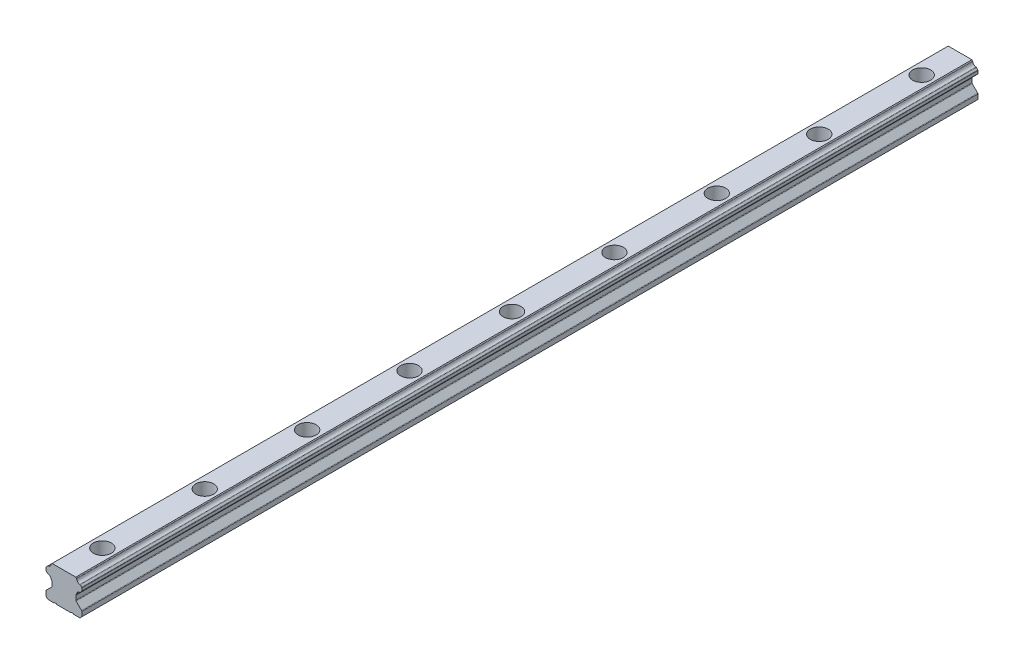
SolidWorks part; units mm, degrees
ref_plane "前视基准面" through (0, 0, 0) normal (0, 0, 1) x (1, 0, 0)
ref_plane "上视基准面" through (0, 0, 0) normal (0, 1, 0) x (1, 0, 0)
ref_plane "右视基准面" through (0, 0, 0) normal (1, 0, 0) x (0, 0, -1)
ref_plane "基准面4" through (0, 0, -110) normal (0, 0, -1) x (-1, 0, 0)
sketch "草图1" plane through (0, 0, -110) normal (0, 0, -1) x (-1, 0, 0)
  line L0 (-14, -4.7442) -> (-14, -26)
  line L1 (-14, -26) -> (14, -26)
  line L2 (14, -26) -> (14, -4.7442)
  line L3 (14, -4.7442) -> (9.2558, 0)
  line L4 (9.2558, 0) -> (-9.2558, 0)
  line L5 (-9.2558, 0) -> (-14, -4.7442)
extrude "凸台-拉伸1" add sketch "草图1" against normal blind 700
sketch "草图2" plane through (0, 0, 590) normal (0, 0, 1) x (1, 0, 0)
  line L0 (14, -7.2617) -> (9.3, -11.9617)
  line L1 (9.3, -11.9617) -> (9.3, -15.8589)
  line L2 (9.3, -15.8589) -> (14, -15.8589)
  line L3 (14, -15.8589) -> (14, -7.2617)
extrude "切除-拉伸1" cut sketch "草图2" against normal through all
sketch "草图3" plane through (0, 0, 590) normal (0, 0, 1) x (1, 0, 0)
  line L0 (9.9011, -11.3606) -> (12.5697, -8.692)
  arc A0 (12.5697, -8.692) -> (9.9011, -11.3606) centre (12.7267, -11.5176) ccw
extrude "切除-拉伸2" cut sketch "草图3" against normal up to next
sketch "草图4" plane through (0, 0, 590) normal (0, 0, 1) x (1, 0, 0)
  line L0 (6.05, -26) -> (7.25, -26)
  line L1 (7.25, -26) -> (7.25, -25.5)
  line L2 (7.25, -25.5) -> (6.05, -25.5)
  line L3 (6.05, -25.5) -> (6.05, -26)
extrude "切除-拉伸3" cut sketch "草图4" against normal through all
sketch "草图5" plane through (0, 0, 590) normal (0, 0, 1) x (1, 0, 0)
  line L0 (-7.25, -26) -> (-6.05, -26)
  line L1 (-6.05, -26) -> (-6.05, -25.5)
  line L2 (-6.05, -25.5) -> (-7.25, -25.5)
  line L3 (-7.25, -25.5) -> (-7.25, -26)
extrude "切除-拉伸4" cut sketch "草图5" against normal through all
sketch "草图6" plane through (0, 0, 590) normal (0, 0, 1) x (1, 0, 0)
  line L0 (-14, -20.5589) -> (-9.3, -20.5589)
  line L1 (-9.3, -20.5589) -> (-9.3, -11.9617)
  line L2 (-9.3, -11.9617) -> (-14, -7.2617)
  line L3 (-14, -7.2617) -> (-14, -20.5589)
extrude "切除-拉伸5" cut sketch "草图6" against normal through all
sketch "草图7" plane through (0, 0, 590) normal (0, 0, 1) x (1, 0, 0)
  line L0 (-12.5697, -8.692) -> (-9.9011, -11.3606)
  arc A0 (-9.9011, -11.3606) -> (-12.5697, -8.692) centre (-12.7267, -11.5176) ccw
extrude "切除-拉伸6" cut sketch "草图7" against normal up to next
sketch "草图8" plane through (0, 0, 590) normal (0, 0, 1) x (1, 0, 0)
  line L0 (-9.9014, -0.6456) -> (-12.5637, -3.3079)
  arc A0 (-12.5637, -3.3079) -> (-9.9014, -0.6456) centre (-12.7267, -0.4826) ccw
extrude "切除-拉伸7" cut sketch "草图8" against normal up to next
sketch "草图9" plane through (0, 0, 590) normal (0, 0, 1) x (1, 0, 0)
  line L0 (12.5637, -3.3079) -> (9.9014, -0.6456)
  arc A0 (9.9014, -0.6456) -> (12.5637, -3.3079) centre (12.7267, -0.4826) ccw
extrude "切除-拉伸8" cut sketch "草图9" against normal up to next
draft "拔模1" type of draft neutral plane draft angle 45 faces to draft 1 face at (11.65, -15.8589, 240) neutral plane through (9.3, -11.9617, -110) neutral plane normal (1, 0, 0) parameters "D1"=45
draft "拔模2" type of draft neutral plane draft angle 45 faces to draft 1 face at (-11.65, -20.5589, 240) neutral plane through (-14, -26, 590) neutral plane normal (-1, 0, 0) parameters "D1"=45
draft "拔模3" type of draft neutral plane draft angle 45 faces to draft 2 face at (6.05, -25.75, 240) face at (7.25, -25.75, 240) neutral plane through (7.25, -25.5, -110) neutral plane normal (0, -1, 0) parameters "D1"=45
draft "拔模4" type of draft neutral plane draft angle 45 faces to draft 2 face at (-7.25, -25.75, 240) face at (-6.05, -25.75, 240) neutral plane through (-6.05, -25.5, -110) neutral plane normal (0, -1, 0) parameters "D1"=45
hole_wizard "M8 六角头螺栓的柱形沉头孔1" positions "草图11" profile "草图10" counterbore size "M8" standard "ANSI Metric"
sketch "草图11" plane through (0, 0, 0) normal (0, 1, 0) x (1, 0, 0)
  point P0 (0, -160)
  point P1 (0, -240)
  point P2 (0, -320)
  point P3 (0, -400)
  point P4 (0, -480)
  point P5 (0, -560)
  point P6 (0, 80)
  point P7 (0, -80)
  point P8 (0, 0)
sketch "草图10" plane through (0, 0, 160) normal (1, 0, 0) x (0, 0, 1)
  line L0 (0, 0) -> (0, 26)
  line L1 (0, 26) -> (4.5, 26)
  line L3 (4.5, 26) -> (4.5, 12)
  line L4 (4.5, 12) -> (7, 12)
  line L5 (7, 12) -> (7, 0)
  line L7 (7, 0) -> (0, 0)
  line L11 (0, -6.35) -> (0, 107.95) construction
  dimension "通孔孔直径" = 9
  dimension "通孔孔深度" = 26
  dimension "柱形沉头孔直径" = 14
  dimension "柱形沉头孔深度" = 12
chamfer "倒角1" distance 1.5 angle 45 2 edges at (-14, -26, 240) (14, -26, 240)
fillet "圆角1" radius 0.6 12 edges at (12.5697, -8.692, 240) (9.9011, -11.3606, 240) (-12.5637, -3.3079, 240) (-9.9014, -0.6456, 240) (14, -4.7442, 240) (-9.9011, -11.3606, 240) (-12.5697, -8.692, 240) (9.9014, -0.6456, 240) (12.5637, -3.3079, 240) (14, -7.2617, 240) (-14, -7.2617, 240) (-14, -4.7442, 240)
fillet "圆角2" radius 0.8 6 edges at (14, -20.5589, 240) (9.3, -11.9617, 240) (9.3, -15.8589, 240) (-9.3, -11.9617, 240) (-14, -20.5589, 240) (-9.3, -15.8589, 240)
